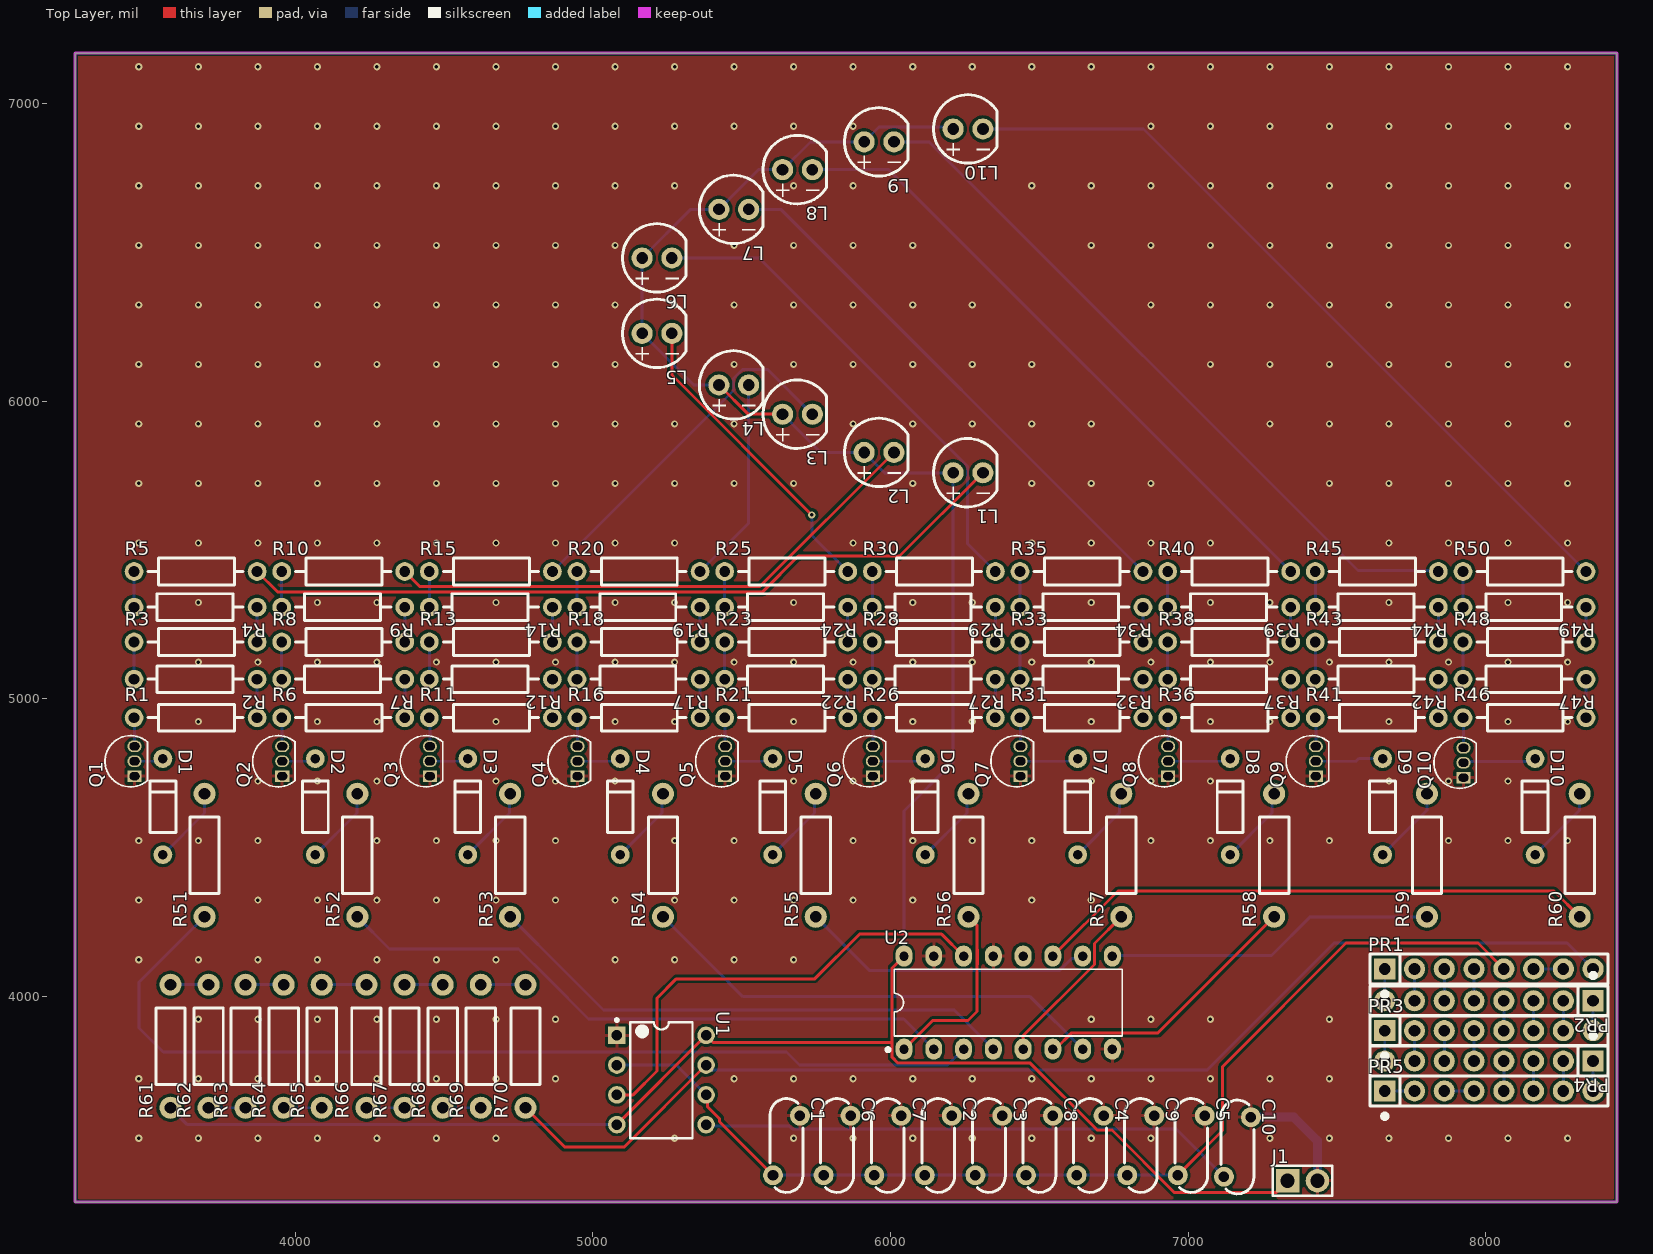
[diagram p0: Top Layer view]
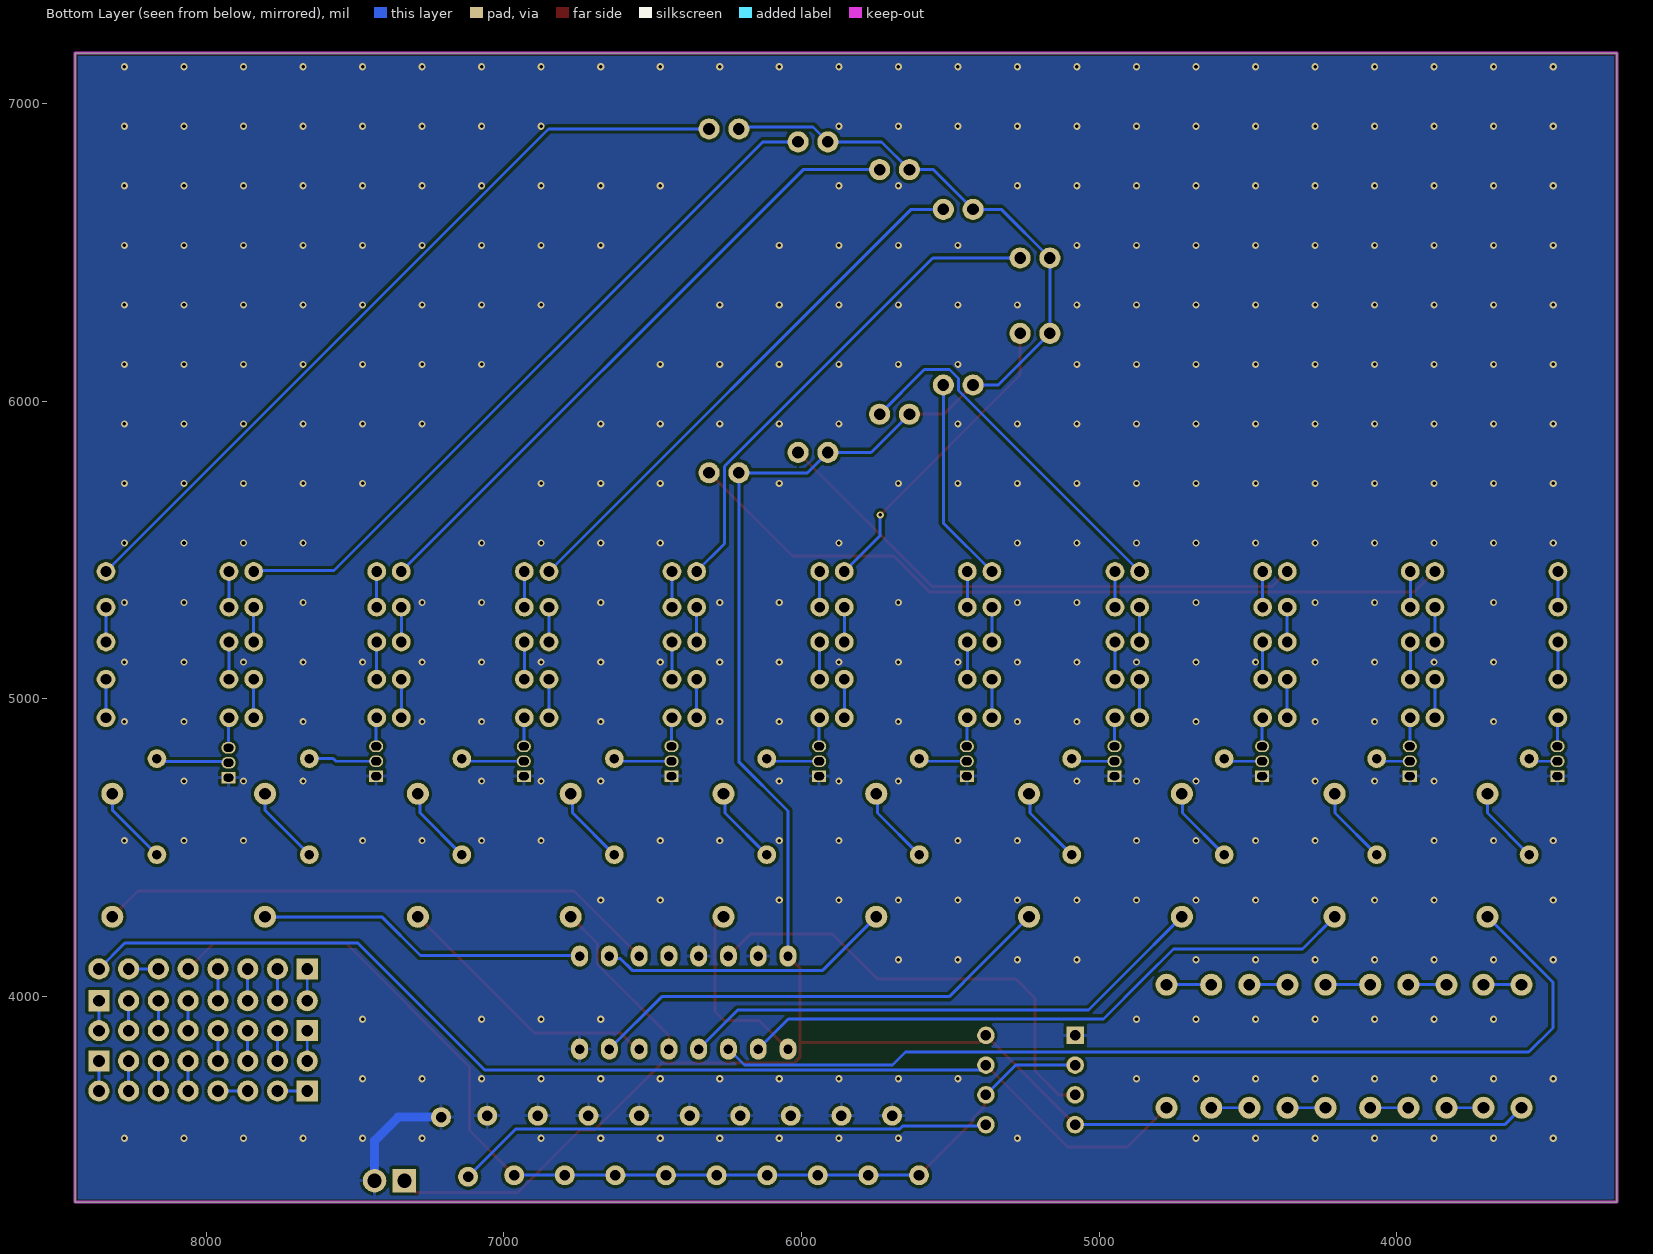
[diagram p1: Bottom Layer view, seen from below]
# Altium PCB MISC51825.pcbdoc
Units mil, origin at the board's own origin, x right, y up, seen from the top; angles counter-clockwise.
Board outline 5180 x 3860 mil, 2 copper layers (Top Layer, Bottom Layer), stack 62.206 mil thick; 118 components, 124 nets, 296 pads, 364 vias.

## Layer stack, top to bottom
Top Solder Mask Layer: solder mask 0.394, Dk 3.3
Top Layer: signal copper 1.379
Dielectric1: surface 59.449, FR4, Dk 4.5
Bottom Layer: signal copper 1.378
Bottom Solder Mask Layer: solder mask 0.394, Dk 3.3

## Board outline
3260,7170 3260,3310 8440,3310 8440,7170

## Design rules (kind name [scope] priority, off if disabled: settings)
BoardOutlineClearance copperThickness2oz_1 [All] p2 off: genericclearance=7.99 ignorepadtopadclearanceinfootprint=FALSE except(0: Arc-SplitContinuation Track-SplitContinuation SMDPad-SplitContinuation THPad-SplitContinuation Via-SplitContinuation Fill-SplitContinuation Region-SplitContinuation Poly-SplitContinuation Text-SplitContinuation Hole-SplitContinuation; 5.98: Arc-CutoutEdge SMDPad-CutoutEdge THPad-CutoutEdge Via-CutoutEdge Fill-CutoutEdge Region-CutoutEdge Text-CutoutEdge; 6.93: Hole-OutlineEdge Hole-CutoutEdge; 10: Poly-OutlineEdge Poly-CutoutEdge; 11.81: Arc-OutlineEdge Track-OutlineEdge SMDPad-OutlineEdge THPad-OutlineEdge Via-OutlineEdge Fill-OutlineEdge Region-OutlineEdge Text-OutlineEdge Track-CutoutEdge)
BoardOutlineClearance Plane_innerPlane_1 [All] p4 off: genericclearance=4.02 ignorepadtopadclearanceinfootprint=FALSE except(0: Arc-SplitContinuation Track-SplitContinuation SMDPad-SplitContinuation THPad-SplitContinuation Via-SplitContinuation Fill-SplitContinuation Region-SplitContinuation Poly-SplitContinuation Text-SplitContinuation Hole-SplitContinuation; 6: SMDPad-CutoutEdge THPad-CutoutEdge Via-CutoutEdge Fill-CutoutEdge Region-CutoutEdge Text-CutoutEdge; 6.93: Hole-OutlineEdge Hole-CutoutEdge; 10: Poly-OutlineEdge Poly-CutoutEdge; 11.8: Arc-OutlineEdge Track-OutlineEdge SMDPad-OutlineEdge THPad-OutlineEdge Via-OutlineEdge Fill-OutlineEdge Region-OutlineEdge Text-OutlineEdge; 11.81: Arc-CutoutEdge Track-CutoutEdge)
BoardOutlineClearance Copper_copperRegion_1 [All] p6 off: genericclearance=4.02 ignorepadtopadclearanceinfootprint=FALSE except(0: Arc-SplitContinuation Track-SplitContinuation SMDPad-SplitContinuation THPad-SplitContinuation Via-SplitContinuation Fill-SplitContinuation Region-SplitContinuation Poly-SplitContinuation Text-SplitContinuation Hole-SplitContinuation; 6: SMDPad-CutoutEdge THPad-CutoutEdge Via-CutoutEdge Fill-CutoutEdge Region-CutoutEdge Text-CutoutEdge; 6.93: Hole-OutlineEdge Hole-CutoutEdge; 10: Poly-OutlineEdge Poly-CutoutEdge; 11.8: Arc-OutlineEdge Track-OutlineEdge SMDPad-OutlineEdge THPad-OutlineEdge Via-OutlineEdge Fill-OutlineEdge Region-OutlineEdge Text-OutlineEdge; 11.81: Arc-CutoutEdge Track-CutoutEdge)
BoardOutlineClearance copperThickness1oz_1 [All] p8: genericclearance=4.02 ignorepadtopadclearanceinfootprint=FALSE except(0: Arc-SplitContinuation Track-SplitContinuation SMDPad-SplitContinuation THPad-SplitContinuation Via-SplitContinuation Fill-SplitContinuation Region-SplitContinuation Poly-SplitContinuation Text-SplitContinuation Hole-SplitContinuation; 6: SMDPad-CutoutEdge THPad-CutoutEdge Via-CutoutEdge Fill-CutoutEdge Region-CutoutEdge Text-CutoutEdge; 6.93: Hole-OutlineEdge Hole-CutoutEdge; 10: Poly-OutlineEdge Poly-CutoutEdge; 11.8: Arc-OutlineEdge Track-OutlineEdge SMDPad-OutlineEdge THPad-OutlineEdge Via-OutlineEdge Fill-OutlineEdge Region-OutlineEdge Text-OutlineEdge; 11.81: Arc-CutoutEdge Track-CutoutEdge)
Clearance copperThickness2oz [All] p1 off: gap=7.99 ignorepadtopadclearanceinfootprint=FALSE except(5.98: SMDPad-Track SMDPad-SMDPad THPad-Track SMDPad-THPad THPad-THPad Track-Via SMDPad-Via THPad-Via Via-Via Fill-Track Region-Track Fill-SMDPad Region-SMDPad Fill-THPad Region-THPad Fill-Via Region-Via Fill-Fill Fill-Region Region-Region Arc-Track Arc-SMDPad Arc-THPad Arc-Via Fill-Arc Region-Arc Arc-Arc Text-Track SMDPad-Text Text-THPad Text-Via Fill-Text Region-Text Arc-Text Text-Text; 6.93: Hole-Track Hole-SMDPad Hole-THPad Hole-Via Fill-Hole Region-Hole Hole-Arc Hole-Text; 10: Poly-Track Poly-SMDPad Poly-THPad Poly-Via Poly-Fill Poly-Region Poly-Poly Poly-Arc Poly-Text Poly-Hole)
Clearance Plane_innerPlane [All] p3 off: gap=4.02 ignorepadtopadclearanceinfootprint=FALSE except(5.98: SMDPad-Track SMDPad-SMDPad THPad-Track SMDPad-THPad THPad-THPad Track-Via SMDPad-Via THPad-Via Via-Via Fill-Track Region-Track Fill-SMDPad Region-SMDPad Fill-THPad Region-THPad Fill-Via Region-Via Fill-Fill Fill-Region Region-Region; 6: Arc-Track Arc-SMDPad Arc-THPad Arc-Via Fill-Arc Region-Arc Arc-Arc Text-Track SMDPad-Text Text-THPad Text-Via Fill-Text Region-Text Arc-Text Text-Text; 6.93: Hole-Track Hole-SMDPad Hole-THPad Hole-Via Fill-Hole Region-Hole Hole-Arc Hole-Text; 10: Poly-Track Poly-SMDPad Poly-THPad Poly-Via Poly-Fill Poly-Region Poly-Poly Poly-Arc Poly-Text Poly-Hole)
Clearance Copper_copperRegion [All] p5 off: gap=4.02 ignorepadtopadclearanceinfootprint=FALSE except(5.98: SMDPad-Track SMDPad-SMDPad THPad-Track SMDPad-THPad THPad-THPad Track-Via SMDPad-Via THPad-Via Via-Via Fill-Track Region-Track Fill-SMDPad Region-SMDPad Fill-THPad Region-THPad Fill-Via Region-Via Fill-Fill Fill-Region Region-Region; 6: Arc-Track Arc-SMDPad Arc-THPad Arc-Via Fill-Arc Region-Arc Arc-Arc Text-Track SMDPad-Text Text-THPad Text-Via Fill-Text Region-Text Arc-Text Text-Text; 6.93: Hole-Track Hole-SMDPad Hole-THPad Hole-Via Fill-Hole Region-Hole Hole-Arc Hole-Text; 10: Poly-Track Poly-SMDPad Poly-THPad Poly-Via Poly-Fill Poly-Region Poly-Poly Poly-Arc Poly-Text Poly-Hole)
Clearance copperThickness1oz [All] p7: gap=4.02 ignorepadtopadclearanceinfootprint=FALSE except(5.98: SMDPad-Track SMDPad-SMDPad THPad-Track SMDPad-THPad THPad-THPad Track-Via SMDPad-Via THPad-Via Via-Via Fill-Track Region-Track Fill-SMDPad Region-SMDPad Fill-THPad Region-THPad Fill-Via Region-Via Fill-Fill Fill-Region Region-Region; 6: Arc-Track Arc-SMDPad Arc-THPad Arc-Via Fill-Arc Region-Arc Arc-Arc Text-Track SMDPad-Text Text-THPad Text-Via Fill-Text Region-Text Arc-Text Text-Text; 6.93: Hole-Track Hole-SMDPad Hole-THPad Hole-Via Fill-Hole Region-Hole Hole-Arc Hole-Text; 10: Poly-Track Poly-SMDPad Poly-THPad Poly-Via Poly-Fill Poly-Region Poly-Poly Poly-Arc Poly-Text Poly-Hole)
DiffPairsRouting differentialPair [All] p1: maxlimit=6 minlimit=6 mostfreqgap=6 toplayer_minwidth=5 toplayer_prefwidth=10 toplayer_maxwidth=100 toplayer_mingap=6 toplayer_prefgap=6 toplayer_maxgap=6 bottomlayer_minwidth=5 bottomlayer_prefwidth=10 bottomlayer_maxwidth=100 bottomlayer_mingap=6 bottomlayer_prefgap=6 bottomlayer_maxgap=6 maxuncoupledlength=10
HoleToHoleClearance otherClearance [All] p1: gap=11.81 allowstackedmicrovias=TRUE
Length netLength [All] p1: minlimit=0 maxlimit=0
PasteMaskExpansion pasteMaskExpansion [All] p1: expansion=0
PlaneConnect innerPlane [All] p1: planeconnectstyle=Relief reliefexpansion=20 reliefentries=4 reliefconductorwidth=10 reliefairgap=10
PolygonConnect copperRegion [All] p1: connectstyle=Relief reliefconductorwidth=10 reliefentries=4 polygonreliefangle="90 Angle" airgapwidth=10 via.connectstyle=Relief via.reliefconductorwidth=10 via.reliefentries=4 via.polygonreliefangle="90 Angle" via.airgapwidth=10
RoutingVias viaSize [All] p1: holewidth=12.01 width=24.02 viastyle="Through Hole" minholewidth=11.81 minwidth=19.68 maxholewidth=248.03 maxwidth=393.7
SolderMaskExpansion solderMaskExpansion [IsVia] p1: expansion=-1000 istentingtop=TRUE
SolderMaskExpansion solderMaskExpansion [All] p2: expansion=2 istentingtop=FALSE
Width copperThickness2oz_2 [All] p1 off: maxlimit=100 minlimit=8 preferedwidth=10
Width copperThickness1oz_2 [All] p2: maxlimit=100 minlimit=5 preferedwidth=10

## Components (designator, comment, footprint, x,y, rotation, side; value= is the part's Value field where it differs from the comment)
C1 "10nF" CAP-TH_L8.0-W2.8-P5.08-D0.6 5650,3500 r270 top
C2 "10nF" CAP-TH_L8.0-W2.8-P5.08-D0.6 6160,3500 r270 top
C3 "10nF" CAP-TH_L8.0-W2.8-P5.08-D0.6 6330,3500 r270 top
C4 "10nF" CAP-TH_L8.0-W2.8-P5.08-D0.6 6670,3500 r270 top
C5 "10nF" CAP-TH_L8.0-W2.8-P5.08-D0.6 7010,3500 r270 top
C6 "10nF" CAP-TH_L8.0-W2.8-P5.08-D0.6 5820,3500 r270 top
C7 "10nF" CAP-TH_L8.0-W2.8-P5.08-D0.6 5990,3500 r270 top
C8 "10nF" CAP-TH_L8.0-W2.8-P5.08-D0.6 6500,3500 r270 top
C9 "10nF" CAP-TH_L8.0-W2.8-P5.08-D0.6 6840,3500 r270 top
C10 "10nF" CAP-TH_L8.0-W2.8-P5.08-D0.6 7165,3495 r270 top
D1 "1N4148TR" DO-35_BD2.0-L4.2-P8.20-D0.5-RD 3555,4638.39 r270 top
D2 "1N4148TR" DO-35_BD2.0-L4.2-P8.20-D0.5-RD 4067.22,4638.39 r270 top
D3 "1N4148TR" DO-35_BD2.0-L4.2-P8.20-D0.5-RD 4579.44,4638.39 r270 top
D4 "1N4148TR" DO-35_BD2.0-L4.2-P8.20-D0.5-RD 5091.67,4638.39 r270 top
D5 "1N4148TR" DO-35_BD2.0-L4.2-P8.20-D0.5-RD 5603.89,4638.39 r270 top
D6 "1N4148TR" DO-35_BD2.0-L4.2-P8.20-D0.5-RD 6116.11,4638.39 r270 top
D7 "1N4148TR" DO-35_BD2.0-L4.2-P8.20-D0.5-RD 6628.33,4638.39 r270 top
D8 "1N4148TR" DO-35_BD2.0-L4.2-P8.20-D0.5-RD 7140.56,4638.39 r270 top
D9 "1N4148TR" DO-35_BD2.0-L4.2-P8.20-D0.5-RD 7652.78,4638.39 r270 top
D10 "1N4148TR" DO-35_BD2.0-L4.2-P8.20-D0.5-RD 8165,4638.39 r270 top
J1 "PZ254V-11-02P" HDR-TH_2P-P2.54-V-M 7383.93,3381.56 r0 top
L1 "XL-502SURD" LED-TH_BD5.9-P2.54-RD_RED 6260,5760 r180 top
L2 "XL-502SURD" LED-TH_BD5.9-P2.54-RD_RED 5961.01,5828.33 r180 top
L3 "XL-502SURD" LED-TH_BD5.9-P2.54-RD_RED 5687.02,5956.67 r180 top
L4 "XL-502SURD" LED-TH_BD5.9-P2.54-RD_RED 5473.03,6055 r180 top
L5 "XL-502SURD" LED-TH_BD5.9-P2.54-RD_RED 5215.05,6228.33 r180 top
L6 "XL-502SURD" LED-TH_BD5.9-P2.54-RD_RED 5215.05,6481.67 r180 top
L7 "XL-502SURD" LED-TH_BD5.9-P2.54-RD_RED 5473.03,6645 r180 top
L8 "XL-502SURD" LED-TH_BD5.9-P2.54-RD_RED 5687.02,6778.33 r180 top
L9 "XL-502SURD" LED-TH_BD5.9-P2.54-RD_RED 5961.01,6871.67 r180 top
L10 "XL-502SURD" LED-TH_BD5.9-P2.54-RD_RED 6260,6915 r180 top
PR1 "10kΩ" RES-ARRAY-TH_8P-L20.3-W2.5-P2.54 8010,4093.09 r0 top
PR2 "10kΩ" RES-ARRAY-TH_8P-L20.3-W2.5-P2.54 8010,3986.11 r180 top
PR3 "10kΩ" RES-ARRAY-TH_8P-L20.3-W2.5-P2.54 8010,3885.62 r0 top
PR4 "10kΩ" RES-ARRAY-TH_8P-L20.3-W2.5-P2.54 8010,3783.65 r180 top
PR5 "10kΩ" RES-ARRAY-TH_8P-L20.3-W2.5-P2.54 8010,3683.16 r0 top
Q1 "S8050" TO-92-3_L4.5-W3.5-P1.27-L 3459.84,4790.8 r90 top
Q2 "S8050" TO-92-3_L4.5-W3.5-P1.27-L 3955.91,4790.8 r90 top
Q3 "S8050" TO-92-3_L4.5-W3.5-P1.27-L 4451.98,4790.8 r90 top
Q4 "S8050" TO-92-3_L4.5-W3.5-P1.27-L 4948.05,4790.8 r90 top
Q5 "S8050" TO-92-3_L4.5-W3.5-P1.27-L 5444.11,4790.8 r90 top
Q6 "S8050" TO-92-3_L4.5-W3.5-P1.27-L 5940.18,4790.8 r90 top
Q7 "S8050" TO-92-3_L4.5-W3.5-P1.27-L 6436.25,4790.8 r90 top
Q8 "S8050" TO-92-3_L4.5-W3.5-P1.27-L 6932.31,4790.8 r90 top
Q9 "S8050" TO-92-3_L4.5-W3.5-P1.27-L 7428.38,4790.8 r90 top
Q10 "S8050" TO-92-3_L4.5-W3.5-P1.27-L 7924.45,4785.8 r90 top
R1 "100Ω" RES-TH_BD2.2-L6.5-P10.50-D0.6 3664.84,4937.09 r0 top
R2 "100Ω" RES-TH_BD2.2-L6.5-P10.50-D0.6 3664.84,5066.43 r180 top
R3 "100Ω" RES-TH_BD2.2-L6.5-P10.50-D0.6 3664.84,5191.55 r0 top
R4 "100Ω" RES-TH_BD2.2-L6.5-P10.50-D0.6 3664.84,5308.56 r180 top
R5 "100Ω" RES-TH_BD2.2-L6.5-P10.50-D0.6 3664.84,5428.24 r0 top
R6 "100Ω" RES-TH_BD2.2-L6.5-P10.50-D0.6 4160.91,4937.09 r0 top
R7 "100Ω" RES-TH_BD2.2-L6.5-P10.50-D0.6 4160.91,5066.43 r180 top
R8 "100Ω" RES-TH_BD2.2-L6.5-P10.50-D0.6 4160.91,5191.55 r0 top
R9 "100Ω" RES-TH_BD2.2-L6.5-P10.50-D0.6 4160.91,5308.56 r180 top
R10 "100Ω" RES-TH_BD2.2-L6.5-P10.50-D0.6 4160.91,5428.24 r0 top
R11 "100Ω" RES-TH_BD2.2-L6.5-P10.50-D0.6 4656.98,4937.09 r0 top
R12 "100Ω" RES-TH_BD2.2-L6.5-P10.50-D0.6 4656.98,5066.43 r180 top
R13 "100Ω" RES-TH_BD2.2-L6.5-P10.50-D0.6 4656.98,5191.55 r0 top
R14 "100Ω" RES-TH_BD2.2-L6.5-P10.50-D0.6 4656.98,5308.56 r180 top
R15 "100Ω" RES-TH_BD2.2-L6.5-P10.50-D0.6 4656.98,5428.24 r0 top
R16 "100Ω" RES-TH_BD2.2-L6.5-P10.50-D0.6 5153.05,4937.09 r0 top
R17 "100Ω" RES-TH_BD2.2-L6.5-P10.50-D0.6 5153.05,5066.43 r180 top
R18 "100Ω" RES-TH_BD2.2-L6.5-P10.50-D0.6 5153.05,5191.55 r0 top
R19 "100Ω" RES-TH_BD2.2-L6.5-P10.50-D0.6 5153.05,5308.56 r180 top
R20 "100Ω" RES-TH_BD2.2-L6.5-P10.50-D0.6 5153.05,5428.24 r0 top
R21 "100Ω" RES-TH_BD2.2-L6.5-P10.50-D0.6 5649.11,4937.09 r0 top
R22 "100Ω" RES-TH_BD2.2-L6.5-P10.50-D0.6 5649.11,5066.43 r180 top
R23 "100Ω" RES-TH_BD2.2-L6.5-P10.50-D0.6 5649.11,5191.55 r0 top
R24 "100Ω" RES-TH_BD2.2-L6.5-P10.50-D0.6 5649.11,5308.56 r180 top
R25 "100Ω" RES-TH_BD2.2-L6.5-P10.50-D0.6 5649.11,5428.24 r0 top
R26 "100Ω" RES-TH_BD2.2-L6.5-P10.50-D0.6 6145.18,4937.09 r0 top
R27 "100Ω" RES-TH_BD2.2-L6.5-P10.50-D0.6 6145.18,5066.43 r180 top
R28 "100Ω" RES-TH_BD2.2-L6.5-P10.50-D0.6 6145.18,5191.55 r0 top
R29 "100Ω" RES-TH_BD2.2-L6.5-P10.50-D0.6 6145.18,5308.56 r180 top
R30 "100Ω" RES-TH_BD2.2-L6.5-P10.50-D0.6 6145.18,5428.24 r0 top
R31 "100Ω" RES-TH_BD2.2-L6.5-P10.50-D0.6 6641.25,4937.09 r0 top
R32 "100Ω" RES-TH_BD2.2-L6.5-P10.50-D0.6 6641.25,5066.43 r180 top
R33 "100Ω" RES-TH_BD2.2-L6.5-P10.50-D0.6 6641.25,5191.55 r0 top
R34 "100Ω" RES-TH_BD2.2-L6.5-P10.50-D0.6 6641.25,5308.56 r180 top
R35 "100Ω" RES-TH_BD2.2-L6.5-P10.50-D0.6 6641.25,5428.24 r0 top
R36 "100Ω" RES-TH_BD2.2-L6.5-P10.50-D0.6 7137.31,4937.09 r0 top
R37 "100Ω" RES-TH_BD2.2-L6.5-P10.50-D0.6 7137.31,5066.43 r180 top
R38 "100Ω" RES-TH_BD2.2-L6.5-P10.50-D0.6 7137.31,5191.55 r0 top
R39 "100Ω" RES-TH_BD2.2-L6.5-P10.50-D0.6 7137.31,5308.56 r180 top
R40 "100Ω" RES-TH_BD2.2-L6.5-P10.50-D0.6 7137.31,5428.24 r0 top
R41 "100Ω" RES-TH_BD2.2-L6.5-P10.50-D0.6 7633.38,4937.09 r0 top
R42 "100Ω" RES-TH_BD2.2-L6.5-P10.50-D0.6 7633.38,5066.43 r180 top
R43 "100Ω" RES-TH_BD2.2-L6.5-P10.50-D0.6 7633.38,5191.55 r0 top
R44 "100Ω" RES-TH_BD2.2-L6.5-P10.50-D0.6 7633.38,5308.56 r180 top
R45 "100Ω" RES-TH_BD2.2-L6.5-P10.50-D0.6 7633.38,5428.24 r0 top
R46 "100Ω" RES-TH_BD2.2-L6.5-P10.50-D0.6 8129.45,4937.09 r0 top
R47 "100Ω" RES-TH_BD2.2-L6.5-P10.50-D0.6 8129.45,5066.43 r180 top
R48 "100Ω" RES-TH_BD2.2-L6.5-P10.50-D0.6 8129.45,5191.55 r0 top
R49 "100Ω" RES-TH_BD2.2-L6.5-P10.50-D0.6 8129.45,5308.56 r180 top
R50 "100Ω" RES-TH_BD2.2-L6.5-P10.50-D0.6 8129.45,5428.24 r0 top
R51 "1kΩ" RES-TH_BD2.5-L6.5-P10.50-D0.6 3695,4475 r90 top
R52 "1kΩ" RES-TH_BD2.5-L6.5-P10.50-D0.6 4208.33,4475 r90 top
R53 "1kΩ" RES-TH_BD2.5-L6.5-P10.50-D0.6 4721.67,4475 r90 top
R54 "1kΩ" RES-TH_BD2.5-L6.5-P10.50-D0.6 5235,4475 r90 top
R55 "1kΩ" RES-TH_BD2.5-L6.5-P10.50-D0.6 5748.33,4475 r90 top
R56 "1kΩ" RES-TH_BD2.5-L6.5-P10.50-D0.6 6261.67,4475 r90 top
R57 "1kΩ" RES-TH_BD2.5-L6.5-P10.50-D0.6 6775,4475 r90 top
R58 "1kΩ" RES-TH_BD2.5-L6.5-P10.50-D0.6 7288.33,4475 r90 top
R59 "1kΩ" RES-TH_BD2.5-L6.5-P10.50-D0.6 7801.67,4475 r90 top
R60 "1kΩ" RES-TH_BD2.5-L6.5-P10.50-D0.6 8315,4475 r90 top
R61 "1kΩ" RES-TH_BD2.5-L6.5-P10.50-D0.6 3580.49,3833.38 r90 top
R62 "1kΩ" RES-TH_BD2.5-L6.5-P10.50-D0.6 3708.6,3833.38 r90 top
R63 "1kΩ" RES-TH_BD2.5-L6.5-P10.50-D0.6 3832.5,3833.38 r90 top
R64 "1kΩ" RES-TH_BD2.5-L6.5-P10.50-D0.6 3960.61,3833.38 r90 top
R65 "1kΩ" RES-TH_BD2.5-L6.5-P10.50-D0.6 4088.72,3833.38 r90 top
R66 "1kΩ" RES-TH_BD2.5-L6.5-P10.50-D0.6 4238.72,3833.38 r90 top
R67 "1kΩ" RES-TH_BD2.5-L6.5-P10.50-D0.6 4366.83,3833.38 r90 top
R68 "1kΩ" RES-TH_BD2.5-L6.5-P10.50-D0.6 4494.94,3833.38 r90 top
R69 "1kΩ" RES-TH_BD2.5-L6.5-P10.50-D0.6 4623.05,3833.38 r90 top
R70 "1kΩ" RES-TH_BD2.5-L6.5-P10.50-D0.6 4773.05,3833.38 r90 top
U1 "NE555P" DIP-8_L9.8-W6.6-P2.54-LS7.6-BL 5230,3720 r270 top
U2 "CD4017CN" PDIP-16_L19.3-W6.4-P2.54-LS7.94-BL 6395,3980 r0 top

## Footprints (in the part's own frame and the unit in brackets; to place one, negate y for a bottom-side part, rotate by r counter-clockwise, add the part's x,y. Pads: shape width x height; smd on the part's side, far side on the other; paste and mask are expansions set on the pad)
CAP-TH_L8.0-W2.8-P5.08-D0.6 [mm]
  round 1.7 hole 0.9 paste+0 mask+0.05: 1(-2.54,1.15) 2(2.54,-1.15)
  silkscreen extent -4,-1.4 4,1.4
DIP-8_L9.8-W6.6-P2.54-LS7.6-BL [mm]
  rect 1.5x1.5 hole 0.9: 1(-3.81,-3.81)
  round 1.5 hole 0.9: 2(-1.27,-3.81) 3(1.27,-3.81) 4(3.81,-3.81) 5(3.81,3.81) 6(1.27,3.81) 7(-1.27,3.81) 8(-3.81,3.81)
  silkscreen extent -5.23,-3.93 4.96,2.65
DO-35_BD2.0-L4.2-P8.20-D0.5-RD [mm]
  round 1.6 hole 0.8: 1(-4.1,0) 2(4.1,0)
  silkscreen extent -2.2,-1.1 2.2,1.1
HDR-TH_2P-P2.54-V-M [mm]
  rect 2x2 hole 1.2: 1(-1.27,0)
  round 2 hole 1.2: 2(1.27,0)
  silkscreen extent -2.54,-1.27 2.54,1.27
LED-TH_BD5.9-P2.54-RD_RED [mm]
  round 1.8 hole 1 paste+0 mask+0.05: 1(-1.27,0) 2(1.27,0)
  silkscreen extent -2.49,-2.92 2.94,2.92
PDIP-16_L19.3-W6.4-P2.54-LS7.94-BL [mm]
  oval 1.44x1.8 hole 0.8: 1(-8.89,-3.97) 2(-6.35,-3.97) 3(-3.81,-3.97) 4(-1.27,-3.97) 5(1.27,-3.97) 6(3.81,-3.97) 7(6.35,-3.97) 8(8.89,-3.97) 9(8.89,3.97) 10(6.35,3.97) 11(3.81,3.97) 12(1.27,3.97) 13(-1.27,3.97) 14(-3.81,3.97) 15(-6.35,3.97) 16(-8.89,3.97)
  silkscreen extent -10.41,-4.17 9.73,2.84
RES-ARRAY-TH_8P-L20.3-W2.5-P2.54 [mm]
  rect 1.8x1.8 hole 1: 1(-8.89,0)
  round 1.8 hole 1: 2(-6.35,0) 3(-3.81,0) 4(-1.27,0) 5(1.27,0) 6(3.81,0) 7(6.35,0) 8(8.89,0)
  silkscreen extent -10.16,-2.36 10.16,1.27
RES-TH_BD2.2-L6.5-P10.50-D0.6 [mm]
  round 1.6 hole 0.914: 1(-5.25,0) 2(5.25,0)
  silkscreen extent -4.06,-1.14 4.06,1.14
RES-TH_BD2.5-L6.5-P10.50-D0.6 [mil]
  round 74 hole 39.37: 1(-206.69,0) 2(206.69,0)
  silkscreen extent -128,-49 128,49
TO-92-3_L4.5-W3.5-P1.27-L [mm]
  rect 1x1.2 hole 0.7 slot 0.85 at 90 deg: 1(-1.27,0)
  oval 1x1.2 hole 0.7 slot 0.85 at 90 deg: 2(0,0) 3(1.27,0)
  silkscreen extent -2.19,-1.1 2.19,2.52

## Via types
v1: diameter 24.02, hole 12, Top Layer to Bottom Layer, 364 vias

## Nets (pads, with @x,y where several pads share a name; then routed paths per layer and width w, separated by ;. In a path a pad name is that pad's centre, name@x,y a point inside that pad or via, vN(x,y) a via of type N, cw(c..) or ccw(c..) an arc to the next point about the centre after c; other vN are vias at no path point)
$1N509: U1.3 U2.14 | length 1562.7
  Top Layer w10: U1.3 5135,3670 5215,3750 5215,3995 5280,4060 5745,4060 5895,4210 6171.3,4210 U2.14
$1N552: C10.2 U1.5 | length 1811.3
  Bottom Layer w10: U1.5 5389.72,3565 5659.72,3565 5669.72,3555 6959.72,3555 C10.2
$1N1039: R60.1 U2.11 | length 1896.5
  Top Layer w10: U2.11 6763.7,4355 8228.31,4355 R60.1
$1N1041: R59.1 U2.9 | length 1110.6
  Bottom Layer w10: U2.9 6761.67,4138.31 7279.71,4138.31 7409.71,4268.31 R59.1
$1N1043: R58.1 U2.6 | length 927.5
  Top Layer w10: U2.6 6553.73,3823.7 6608.34,3878.31 6898.34,3878.31 R58.1
$1N1045: R57.1 U2.5 | length 581.3
  Top Layer w10: U2.5 6445,3868.31 6685,4108.31 6685,4178.31 R57.1
$1N1047: R56.1 U2.1 | length 692.2
  Top Layer w10: R56.1 6290,4239.98 6290,4159.98 ; U2.1@6051.67,3830.37 6051.67,3828.31 U2.1 U2.1@6051.67,3830.37 ; U2.1@6051.67,3830.37 6141.3,3920 6260,3920 6290,3950 6290,4106.64 ; 6290,4106.64 6290,4159.98 ; 6290,4106.64 6291.67,4108.31 6291.67,4158.31 6290,4159.98
$1N1049: R55.1 U2.10 | length 989.6
  Bottom Layer w10: R55.1 5928.33,4088.31 6568.33,4088.31 6608.33,4128.31 6628.33,4128.31 U2.10
$1N1051: R54.1 U2.7 | length 1594.2
  Bottom Layer w10: R54.1 5402.89,4100.42 5503.31,4000 6468.7,4000 U2.7
$1N1053: R53.1 U2.4 | length 1807.5
  Bottom Layer w10: R53.1 4912.26,4077.72 5034.98,3955 6213.7,3955 U2.4
$1N1055: R51.1 U2.3 | length 3308.5
  Bottom Layer w10: R51.1 3475,4048.31 3475,3895 3556.3,3813.7 5650.32,3813.7 5694.02,3770 6191.3,3770 U2.3
$1N1057: R52.1 U2.2 | length 2120.8
  Bottom Layer w10: R52.1 4316.64,4160 4750,4160 4847.69,4062.31 4985,3925 6043.7,3925 U2.2
$1N1689: R4.2 R5.1 | length 119.7
  Bottom Layer w10: R4.2@3458.15,5308.56 R5.1
$1N1693: R3.2 R4.1 | length 117
  Bottom Layer w10: R3.2 R4.1
$1N1698: R2.2 R3.1 | length 125.1
  Bottom Layer w10: R2.2@3458.15,5066.43 R3.1
$1N1703: R1.2 R2.1 | length 129.3
  Bottom Layer w10: R1.2 R2.1
$1N1886: R6.2 R7.1 | length 129.3
  Bottom Layer w10: R6.2 R7.1
$1N1888: R8.2 R9.1 | length 117
  Bottom Layer w10: R8.2 R9.1
$1N1890: R7.2 R8.1 | length 125.1
  Bottom Layer w10: R7.2 R8.1
$1N1892: R9.2 R10.1 | length 119.7
  Bottom Layer w10: R9.2 R10.1
$1N2074: R11.2 R12.1 | length 129.3
  Bottom Layer w10: R11.2 R12.1
$1N2076: R13.2 R14.1 | length 117
  Bottom Layer w10: R13.2 R14.1
$1N2078: R12.2 R13.1 | length 125.1
  Bottom Layer w10: R12.2 R13.1
$1N2080: R14.2 R15.1 | length 119.7
  Bottom Layer w10: R14.2 R15.1
$1N2826: R16.2 R17.1 | length 129.3
  Bottom Layer w10: R16.2 R17.1
$1N2828: R18.2 R19.1 | length 117
  Bottom Layer w10: R18.2 R19.1
$1N2830: R17.2 R18.1 | length 125.1
  Bottom Layer w10: R17.2@4946.35,5066.43 R18.1@4946.35,5191.54
$1N2832: R19.2 R20.1 | length 119.7
  Bottom Layer w10: R19.2@4946.35,5308.56 R20.1@4946.35,5428.24
$1N3014: R21.2 R22.1 | length 129.3
  Bottom Layer w10: R21.2 R22.1
$1N3016: R23.2 R24.1 | length 117
  Bottom Layer w10: R23.2 R24.1
$1N3018: R22.2 R23.1 | length 125.1
  Bottom Layer w10: R22.2 R23.1
$1N3020: R24.2 R25.1 | length 119.7
  Bottom Layer w10: R24.2 R25.1
$1N4862: R32.2 R33.1 | length 125.1
  Bottom Layer w10: R32.2@6434.55,5066.43 R33.1@6434.55,5191.54
$1N4864: R33.2 R34.1 | length 117
  Bottom Layer w10: R33.2 R34.1
$1N4866: R31.2 R32.1 | length 129.3
  Bottom Layer w10: R31.2 R32.1
$1N4868: R34.2 R35.1 | length 119.7
  Bottom Layer w10: R34.2@6434.55,5308.56 R35.1@6434.55,5428.24
$1N4870: R26.2 R27.1 | length 129.3
  Bottom Layer w10: R26.2 R27.1
$1N4872: R27.2 R28.1 | length 125.1
  Bottom Layer w10: R27.2 R28.1
$1N4874: R28.2 R29.1 | length 117
  Bottom Layer w10: R28.2 R29.1
$1N4876: R29.2 R30.1 | length 119.7
  Bottom Layer w10: R29.2 R30.1
$1N4878: R37.2 R38.1 | length 125.1
  Bottom Layer w10: R37.2 R38.1
$1N4880: R39.2 R40.1 | length 119.7
  Bottom Layer w10: R39.2 R40.1
$1N4882: R36.2 R37.1 | length 129.3
  Bottom Layer w10: R36.2 R37.1
$1N4884: R38.2 R39.1 | length 117
  Bottom Layer w10: R38.2 R39.1
$1N4886: R47.2 R48.1 | length 125.1
  Bottom Layer w10: R47.2 R48.1
$1N4888: R48.2 R49.1 | length 117
  Bottom Layer w10: R48.2 R49.1
$1N4890: R46.2 R47.1 | length 129.3
  Bottom Layer w10: R46.2 R47.1
$1N4892: R49.2 R50.1 | length 119.7
  Bottom Layer w10: R49.2 R50.1
$1N4894: R44.2 R45.1 | length 119.7
  Bottom Layer w10: R44.2 R45.1
$1N4896: R43.2 R44.1 | length 117
  Bottom Layer w10: R43.2 R44.1
$1N4898: R42.2 R43.1 | length 125.1
  Bottom Layer w10: R42.2 R43.1
$1N4900: R41.2 R42.1 | length 129.3
  Bottom Layer w10: R41.2 R42.1
$1N6278: D1.2 R51.2 | length 262.7
  Bottom Layer w10: D1.2 3695,4616.97 R51.2
$1N6282: D2.2 R52.2 | length 262.8
  Bottom Layer w10: D2.2 4207.22,4616.97 4207.22,4666.97 R52.2
$1N6287: D3.2 R53.2 | length 262.9
  Bottom Layer w10: D3.2 4719.44,4616.97 4719.44,4666.97 R53.2
$1N6292: D4.2 R54.2 | length 263.1
  Bottom Layer w10: D4.2 5231.67,4616.97 5231.67,4666.97 R54.2
$1N6297: D5.2 R55.2 | length 263.4
  Bottom Layer w10: D5.2 5743.89,4616.97 5743.89,4666.97 R55.2
$1N6302: D6.2 R56.2 | length 263.7
  Bottom Layer w10: D6.2 6256.11,4616.97 6256.11,4666.97 R56.2
$1N6307: D7.2 R57.2 | length 264.2
  Bottom Layer w10: D7.2 6768.33,4616.97 6768.33,4666.97 R57.2
$1N6312: D8.2 R58.2 | length 264.6
  Bottom Layer w10: D8.2 7280.56,4616.97 7280.56,4666.97 R58.2
$1N6317: D9.2 R59.2 | length 266.4
  Bottom Layer w10: D9.2 7801.67,4625.86 R59.2
$1N6322: D10.2 R60.2 | length 266.9
  Bottom Layer w10: D10.2 8315,4626.97 R60.2
$1N6789: Q10.3 R46.1 | length 102
  Bottom Layer w10: R46.1 7924.45,4935.4 Q10.3
$1N6799: Q9.3 R41.1 | length 97
  Bottom Layer w10: R41.1 7426.69,4932.5 7428.38,4930.8 Q9.3
$1N6801: Q8.3 R36.1 | length 96.5
  Bottom Layer w10: R36.1 6932.31,4930.8 Q8.3
$1N6803: Q7.3 R31.1 | length 96.5
  Bottom Layer w10: R31.1@6434.55,4937.09 6436.25,4930.8 Q7.3
$1N6805: Q6.3 R26.1 | length 96.5
  Bottom Layer w10: R26.1 5940.18,4930.8 Q6.3
$1N6807: Q5.3 R21.1 | length 96.5
  Bottom Layer w10: R21.1 5444.11,4930.8 Q5.3
$1N6809: Q4.3 R16.1 | length 96.5
  Bottom Layer w10: R16.1@4946.35,4937.09 4948.04,4930.8 Q4.3
$1N6811: Q3.3 R11.1 | length 97
  Bottom Layer w10: R11.1 4450.28,4932.5 4451.98,4930.8 Q3.3
$1N6813: Q2.3 R6.1 | length 96.5
  Bottom Layer w10: R6.1 3955.91,4930.8 Q2.3
$1N6815: Q1.3 R1.1 | length 96.5
  Bottom Layer w10: R1.1 3459.84,4930.8 Q1.3
$1N6819: D1.1 Q1.2 | length 98.9
  Bottom Layer w10: Q1.2 3525.99,4790.8 3535,4799.81 D1.1
$1N6827: D2.1 Q2.2 | length 115
  Bottom Layer w10: Q2.2 4038.22,4790.8 4047.22,4799.81 D2.1
$1N6833: D3.1 Q3.2 | length 131.2
  Bottom Layer w10: Q3.2 4560.43,4790.8 4569.44,4799.81 D3.1
$1N6840: D4.1 Q4.2 | length 147.4
  Bottom Layer w10: Q4.2 5072.66,4790.8 5081.67,4799.81 D4.1
$1N6847: D5.1 Q5.2 | length 163.5
  Bottom Layer w10: Q5.2 5584.88,4790.8 5593.89,4799.81 D5.1
$1N6854: D6.1 Q6.2 | length 179.7
  Bottom Layer w10: Q6.2 6107.1,4790.8 D6.1
$1N6860: D7.1 Q7.2 | length 195.8
  Bottom Layer w10: Q7.2 6619.32,4790.8 D7.1
$1N6867: D8.1 Q8.2 | length 212
  Bottom Layer w10: Q8.2 7131.55,4790.8 D8.1
$1N6874: D9.1 Q9.2 | length 228.1
  Bottom Layer w10: Q9.2 7563.77,4790.8 7572.78,4799.81 D9.1
$1N6881: D10.1 Q10.2 | length 245.4
  Bottom Layer w10: Q10.2 7935,4789.81 8155,4789.81 D10.1
$1N7123: L1.1 R5.2 | length 2632.4
  Top Layer w10: R5.2 3939.78,5360 5570,5360 5690,5480 6030,5480 L1.1
$1N7169: L2.1 R10.2 | length 1850.5
  Top Layer w10: R10.2 4417.51,5378.34 5561.01,5378.34 L2.1
$1N7259: L3.1 R15.2 | length 1239.9
  Bottom Layer w10: R15.2 5472.1,6036.67 5472.1,6076.67 5502.1,6106.66 5587.02,6106.66 L3.1
$1N7261: L4.1 R20.2 | length 694.4
  Bottom Layer w10: R20.2 5523.03,5591.53 L4.1
$1N7351: L5.1 R25.2 | length 1044.8
  Top Layer w10: L5.1 5265.05,6088.33 v1(5735.05,5618.34)
  Bottom Layer w10: v1(5735.05,5618.34) 5735.05,5549 R25.2
$1N7353: L6.1 R30.2 | length 1675.5
  Bottom Layer w10: L6.1 5558.45,6481.67 6258.45,5781.67 6258.45,5521.67 R30.2
$1N7443: L7.1 R35.2 | length 1828.9
  Bottom Layer w10: L7.1 5631.18,6645 R35.2
$1N7445: L8.1 R40.2 | length 2166.2
  Bottom Layer w10: L8.1 5993.92,6778.33 R40.2
$1N7535: L9.1 R45.2 | length 2427
  Bottom Layer w10: L9.1 6129.75,6871.67 7569.75,5431.67 7836.65,5431.67 R45.2
$1N7537: L10.1 R50.2 | length 2642
  Bottom Layer w10: L10.1 6849.39,6915 R50.2
$1N8324: PR5.1 PR5.2 | length 100
  Bottom Layer w10: PR5.1 PR5.2
$1N8328: PR5.3 PR5.4 | length 100
  Bottom Layer w10: PR5.3 PR5.4
$1N8333: PR4.1 PR5.8 | length 100.5
  Bottom Layer w10: PR5.8 PR4.1
$1N8338: PR4.2 PR5.7 | length 100.5
  Bottom Layer w10: PR5.7 PR4.2
$1N8343: PR4.3 PR5.6 | length 100.5
  Bottom Layer w10: PR5.6 PR4.3
$1N8348: PR4.4 PR5.5 | length 100.5
  Bottom Layer w10: PR5.5 PR4.4
$1N8353: PR3.4 PR4.5 | length 102
  Bottom Layer w10: PR4.5 PR3.4
$1N8358: PR3.3 PR4.6 | length 102
  Bottom Layer w10: PR4.6 PR3.3
$1N8363: PR3.2 PR4.7 | length 102
  Bottom Layer w10: PR4.7 PR3.2
$1N8368: PR3.1 PR4.8 | length 102
  Bottom Layer w10: PR4.8 PR3.1
$1N8379: PR2.1 PR3.8 | length 100.5
  Bottom Layer w10: PR3.8 PR2.1
$1N8383: PR2.2 PR3.7 | length 100.5
  Bottom Layer w10: PR3.7 PR2.2
$1N8388: PR2.3 PR3.6 | length 100.5
  Bottom Layer w10: PR3.6 PR2.3
$1N8393: PR2.4 PR3.5 | length 100.5
  Bottom Layer w10: PR3.5 PR2.4
$1N8398: PR1.4 PR2.5 | length 107
  Bottom Layer w10: PR2.5 PR1.4
$1N8403: PR1.3 PR2.6 | length 107
  Bottom Layer w10: PR2.6 PR1.3
$1N8408: PR1.2 PR2.7 | length 107
  Bottom Layer w10: PR2.7 PR1.2
$1N8413: PR1.1 PR2.8 | length 107
  Bottom Layer w10: PR2.8 PR1.1
$1N8418: PR1.6 PR1.7 | length 100
  Bottom Layer w10: PR1.6 PR1.7
$1N8423: C1.2 C2.2 C3.2 C4.2 C5.2 C6.2 C7.2 C8.2 C9.2 PR1.5 U1.2 U1.6 | length 3649.9
  Top Layer w10: U1.6 5384.72,3660 5384.72,3630 5424.72,3590 5424.72,3580 C1.2 ; C5.2 7114.72,3550 7114.72,3764.72 7530,4180 7973.09,4180 PR1.5 PR1.5@8054.72,4090
  Bottom Layer w10: U1.2 5280,3770 U1.6 ; C1.2 C6.2 C7.2 C2.2 C3.2 C8.2 C4.2 C9.2 C5.2
$1N8954: R61.2 R62.2 | length 128.1
  Bottom Layer w10: R61.2 R62.2
$1N8960: R62.1 R63.1 | length 123.9
  Bottom Layer w10: R62.1 R63.1
$1N8967: R63.2 R64.2 | length 128.1
  Bottom Layer w10: R63.2 R64.2
$1N8974: R64.1 R65.1 | length 128.1
  Bottom Layer w10: R64.1 R65.1
$1N8979: R66.1 R67.1 | length 128.1
  Bottom Layer w10: R66.1 R67.1
$1N8983: R68.1 R69.1 | length 128.1
  Bottom Layer w10: R68.1 R69.1
$1N8987: R65.2 R66.2 | length 150
  Bottom Layer w10: R65.2 R66.2
$1N8991: R67.2 R68.2 | length 128.1
  Bottom Layer w10: R67.2 R68.2
$1N8995: R69.2 R70.2 | length 150
  Bottom Layer w10: R69.2 R70.2
$1N9001: PR1.8 R70.1 U1.7 | length 3975.2
  Top Layer w10: R70.1 4904.74,3495 5105,3495 U1.7
  Bottom Layer w10: U1.7 5396.91,3753.09 6692.68,3753.09 7063.13,3753.09 7490.04,4180 8273.08,4180 PR1.8
GND: C1.1 C2.1 C3.1 C4.1 C5.1 C6.1 C7.1 C8.1 C9.1 C10.1 J1.2 Q1.1 Q2.1 Q3.1 Q4.1 Q5.1 Q6.1 Q7.1 Q8.1 Q9.1 Q10.1 U1.1 U2.8 U2.13 U2.15 | length 390.9
  Bottom Layer w30: C10.1 7355,3595 7433.93,3516.07 J1.2
  other v1: 3474.1,3524.1 3674.1,3524.1 3874.1,3524.1 4074.1,3524.1 4274.1,3524.1 4474.1,3524.1 4674.1,3524.1 5274.1,3524.1 5674.1,3524.1 5874.1,3524.1 6074.1,3524.1 6274.1,3524.1 6474.1,3524.1 6674.1,3524.1 6874.1,3524.1 7274.1,3524.1 7474.1,3524.1 7674.1,3524.1 7874.1,3524.1 8074.1,3524.1 8274.1,3524.1 3474.1,3724.1 3674.1,3724.1 3874.1,3724.1 4074.1,3724.1 4274.1,3724.1 4474.1,3724.1 4674.1,3724.1 4874.1,3724.1 5474.1,3724.1 5674.1,3724.1 5874.1,3724.1 6074.1,3724.1 6274.1,3724.1 6474.1,3724.1 6674.1,3724.1 6874.1,3724.1 7074.1,3724.1 7274.1,3724.1 7474.1,3724.1 3674.1,3924.1 3874.1,3924.1 4074.1,3924.1 4274.1,3924.1 4474.1,3924.1 4674.1,3924.1 4874.1,3924.1 6674.1,3924.1 6874.1,3924.1 7074.1,3924.1 7474.1,3924.1 3474.1,4124.1 3674.1,4124.1 3874.1,4124.1 4074.1,4124.1 4274.1,4124.1 4474.1,4124.1 4674.1,4124.1 5074.1,4124.1 5274.1,4124.1 5474.1,4124.1 5674.1,4124.1 3474.1,4324.1 3874.1,4324.1 4074.1,4324.1 4274.1,4324.1 4474.1,4324.1 4674.1,4324.1 4874.1,4324.1 5074.1,4324.1 5274.1,4324.1 5474.1,4324.1 5674.1,4324.1 5874.1,4324.1 6074.1,4324.1 6474.1,4324.1 6674.1,4324.1 3474.1,4524.1 3674.1,4524.1 3874.1,4524.1 4274.1,4524.1 4474.1,4524.1 4674.1,4524.1 4874.1,4524.1 5274.1,4524.1 5474.1,4524.1 5874.1,4524.1 6074.1,4524.1 6274.1,4524.1 6474.1,4524.1 6874.1,4524.1 7074.1,4524.1 7274.1,4524.1 7474.1,4524.1 7874.1,4524.1 8074.1,4524.1 8274.1,4524.1 3874.1,4724.1 4074.1,4724.1 4274.1,4724.1 4674.1,4724.1 4874.1,4724.1 5074.1,4724.1 5674.1,4724.1 5874.1,4724.1 6074.1,4724.1 6674.1,4724.1 6874.1,4724.1 7074.1,4724.1 7674.1,4724.1 7874.1,4724.1 8074.1,4724.1 3674.1,4924.1 4074.1,4924.1 4274.1,4924.1 4674.1,4924.1 5074.1,4924.1 5274.1,4924.1 5674.1,4924.1 6074.1,4924.1 6274.1,4924.1 6674.1,4924.1 7074.1,4924.1 7274.1,4924.1 7674.1,4924.1 8074.1,4924.1 8274.1,4924.1 3674.1,5124.1 3874.1,5124.1 4074.1,5124.1 4274.1,5124.1 4474.1,5124.1 4674.1,5124.1 4874.1,5124.1 5074.1,5124.1 5274.1,5124.1 5474.1,5124.1 5674.1,5124.1 5874.1,5124.1 6074.1,5124.1 6274.1,5124.1 6474.1,5124.1 6674.1,5124.1 6874.1,5124.1 7074.1,5124.1 7274.1,5124.1 7474.1,5124.1 7674.1,5124.1 7874.1,5124.1 8074.1,5124.1 8274.1,5124.1 3674.1,5324.1 4074.1,5324.1 4274.1,5324.1 4674.1,5324.1 5074.1,5324.1 5274.1,5324.1 5674.1,5324.1 6074.1,5324.1 6274.1,5324.1 6674.1,5324.1 7074.1,5324.1 7274.1,5324.1 7674.1,5324.1 8074.1,5324.1 8274.1,5324.1 3474.1,5524.1 3674.1,5524.1 3874.1,5524.1 4074.1,5524.1 4274.1,5524.1 4474.1,5524.1 4674.1,5524.1 4874.1,5524.1 5074.1,5524.1 5274.1,5524.1 5874.1,5524.1 6474.1,5524.1 6674.1,5524.1 6874.1,5524.1 7074.1,5524.1 7674.1,5524.1 7874.1,5524.1 8074.1,5524.1 8274.1,5524.1 3474.1,5724.1 3674.1,5724.1 3874.1,5724.1 4074.1,5724.1 4274.1,5724.1 4474.1,5724.1 4674.1,5724.1 4874.1,5724.1 5074.1,5724.1 5274.1,5724.1 5474.1,5724.1 5674.1,5724.1 6074.1,5724.1 6474.1,5724.1 6674.1,5724.1 6874.1,5724.1 7474.1,5724.1 7674.1,5724.1 7874.1,5724.1 8074.1,5724.1 8274.1,5724.1 3474.1,5924.1 3674.1,5924.1 3874.1,5924.1 4074.1,5924.1 4274.1,5924.1 4474.1,5924.1 4674.1,5924.1 4874.1,5924.1 5074.1,5924.1 5274.1,5924.1 5474.1,5924.1 5874.1,5924.1 6074.1,5924.1 6274.1,5924.1 6474.1,5924.1 6674.1,5924.1 7274.1,5924.1 7474.1,5924.1 7674.1,5924.1 7874.1,5924.1 8074.1,5924.1 8274.1,5924.1 3474.1,6124.1 3674.1,6124.1 3874.1,6124.1 4074.1,6124.1 4274.1,6124.1 4474.1,6124.1 4674.1,6124.1 4874.1,6124.1 5074.1,6124.1 5474.1,6124.1 5674.1,6124.1 5874.1,6124.1 6074.1,6124.1 6274.1,6124.1 6474.1,6124.1 7074.1,6124.1 7274.1,6124.1 7474.1,6124.1 7674.1,6124.1 7874.1,6124.1 8074.1,6124.1 8274.1,6124.1 3474.1,6324.1 3674.1,6324.1 3874.1,6324.1 4074.1,6324.1 4274.1,6324.1 4474.1,6324.1 4674.1,6324.1 4874.1,6324.1 5074.1,6324.1 5274.1,6324.1 5474.1,6324.1 5674.1,6324.1 5874.1,6324.1 6074.1,6324.1 6274.1,6324.1 6874.1,6324.1 7074.1,6324.1 7274.1,6324.1 7474.1,6324.1 7674.1,6324.1 7874.1,6324.1 8074.1,6324.1 8274.1,6324.1 3474.1,6524.1 3674.1,6524.1 3874.1,6524.1 4074.1,6524.1 4274.1,6524.1 4474.1,6524.1 4674.1,6524.1 4874.1,6524.1 5074.1,6524.1 5474.1,6524.1 5674.1,6524.1 5874.1,6524.1 6074.1,6524.1 6674.1,6524.1 6874.1,6524.1 7074.1,6524.1 7274.1,6524.1 7474.1,6524.1 7674.1,6524.1 7874.1,6524.1 8074.1,6524.1 8274.1,6524.1 3474.1,6724.1 3674.1,6724.1 3874.1,6724.1 4074.1,6724.1 4274.1,6724.1 4474.1,6724.1 4674.1,6724.1 4874.1,6724.1 5074.1,6724.1 5274.1,6724.1 5674.1,6724.1 5874.1,6724.1 6474.1,6724.1 6674.1,6724.1 6874.1,6724.1 7074.1,6724.1 7274.1,6724.1 7474.1,6724.1 7674.1,6724.1 7874.1,6724.1 8074.1,6724.1 8274.1,6724.1 3474.1,6924.1 3674.1,6924.1 3874.1,6924.1 4074.1,6924.1 4274.1,6924.1 4474.1,6924.1 4674.1,6924.1 4874.1,6924.1 5074.1,6924.1 5274.1,6924.1 5474.1,6924.1 5674.1,6924.1 5874.1,6924.1 6874.1,6924.1 7074.1,6924.1 7274.1,6924.1 7474.1,6924.1 7674.1,6924.1 7874.1,6924.1 8074.1,6924.1 8274.1,6924.1 3474.1,7124.1 3674.1,7124.1 3874.1,7124.1 4074.1,7124.1 4274.1,7124.1 4474.1,7124.1 4674.1,7124.1 4874.1,7124.1 5074.1,7124.1 5274.1,7124.1 5474.1,7124.1 5674.1,7124.1 5874.1,7124.1 6074.1,7124.1 6274.1,7124.1 6474.1,7124.1 6674.1,7124.1 6874.1,7124.1 7074.1,7124.1 7274.1,7124.1 7474.1,7124.1 7674.1,7124.1 7874.1,7124.1 8074.1,7124.1 8274.1,7124.1
VCC: J1.1 L1.2 L2.2 L3.2 L4.2 L5.2 L6.2 L7.2 L8.2 L9.2 L10.2 R61.1 U1.4 U1.8 U2.16 | length 8886.8
  Top Layer w10: U1.4 U1.8 5403.7,3846.3 6005,3846.3 ; L4.2 5521.36,5956.67 L3.2 ; U2.16 6005,4096.3 6005,3846.3 ; J1.1 7293.93,3341.56 6953.93,3341.56 6743.93,3551.56 6693.93,3551.56 6469.18,3776.3 6025,3776.3 6005,3796.3 6005,3846.3
  Bottom Layer w10: R61.1 3637.17,3570 U1.4 ; L4.2 5338.38,6055 L5.2 L6.2 5328.38,6645 L7.2 5556.36,6778.33 L8.2 5730.35,6871.67 L9.2 5961.01,6921.67 6203.33,6921.67 L10.2 ; L3.2 5765.35,5828.33 L2.2 5979.35,5760 L1.2 6210,4788.78 6045,4623.78 U2.16
pads on no net: U2.12

## Polygon pours and split planes (outlines as drawn)
GND on Bottom Layer (solid, remove dead copper, pour order 2): 3190,7865 3190,3130 8690,3130 8690,7865
GND on Top Layer (solid, remove dead copper, pour order 0): 3000,7730 3000,3000 8835,3000 8835,7730

## Keep-outs
Board Outline Layer:
  the board outline again, w10